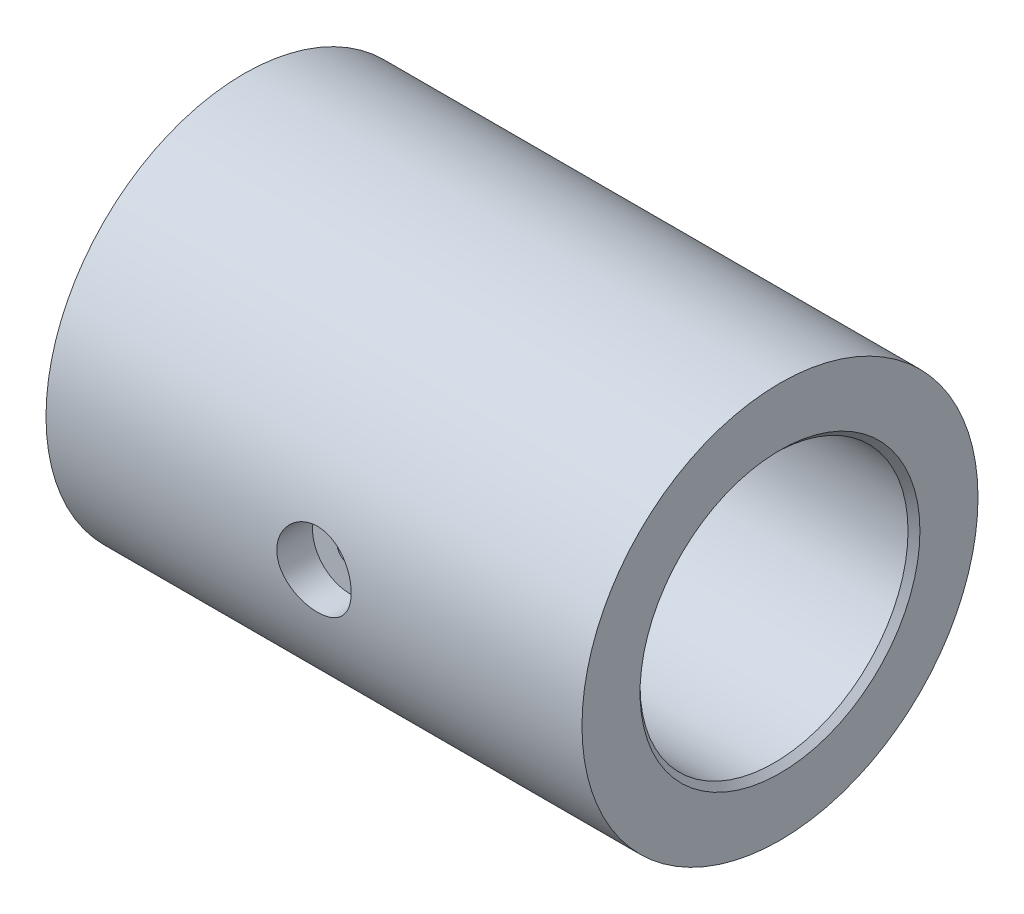
SolidWorks part; units mm, degrees
material "Q345B"
ref_plane "Front Plane" through (0, 0, 0) normal (0, 0, 1) x (1, 0, 0)
ref_plane "Top Plane" through (0, 0, 0) normal (0, 1, 0) x (1, 0, 0)
ref_plane "Right Plane" through (0, 0, 0) normal (1, 0, 0) x (0, 0, -1)
sketch "Sketch1" plane through (0, 0, 0) normal (1, 0, 0) x (0, 0, -1)
  circle A0 centre (0, 0) radius 45
  circle A1 centre (0, 0) radius 66.5
  dimension "D1" = 133
  dimension "D2" = 90
extrude "Boss-Extrude1" add sketch "Sketch1" along normal mid plane 180
ref_plane "Plane1" through (0, 0, 66.5) normal (0, 0, 1) x (1, 0, 0)
hole_wizard "M10 Tapped Hole1" positions "Sketch3" profile "Sketch2" tap size "M10" standard "GB"
sketch "Sketch3" plane through (0, 0, 66.5) normal (0, 0, 1) x (1, 0, 0)
  point P0 (0, 0)
sketch "Sketch2" plane through (0, 0, 66.5) normal (1, 0, 0) x (0, -1, 0)
  line L0 (0, 0) -> (0, 69.0527)
  line L1 (0, 69.0527) -> (4.25, 66.499)
  line L2 (4.25, 66.499) -> (4.25, 0)
  line L5 (4.25, 0) -> (0, 0)
  line L10 (0, 69.0527) -> (-4.25, 66.499) construction
  line L11 (0, -6.35) -> (0, 107.95) construction
  dimension "螺纹孔钻头直径" = 8.5
  dimension "螺纹孔钻头深度" = 66.499
  dimension "导头角度" = 118
cosmetic thread "Cosmetic thread1" parameters "D1"=21.7011, "D2"=10
sketch "Sketch4" plane through (0, 0, 66.5) normal (0, 0, 1) x (1, 0, 0)
  circle A0 centre (0, 0) radius 12.5
  dimension "D1" = 25
extrude "Cut-Extrude1" cut sketch "Sketch4" against normal blind 12
chamfer "Chamfer1" distance 2 angle 45 2 edges at (-90, 0, -45) (90, 0, -45)
